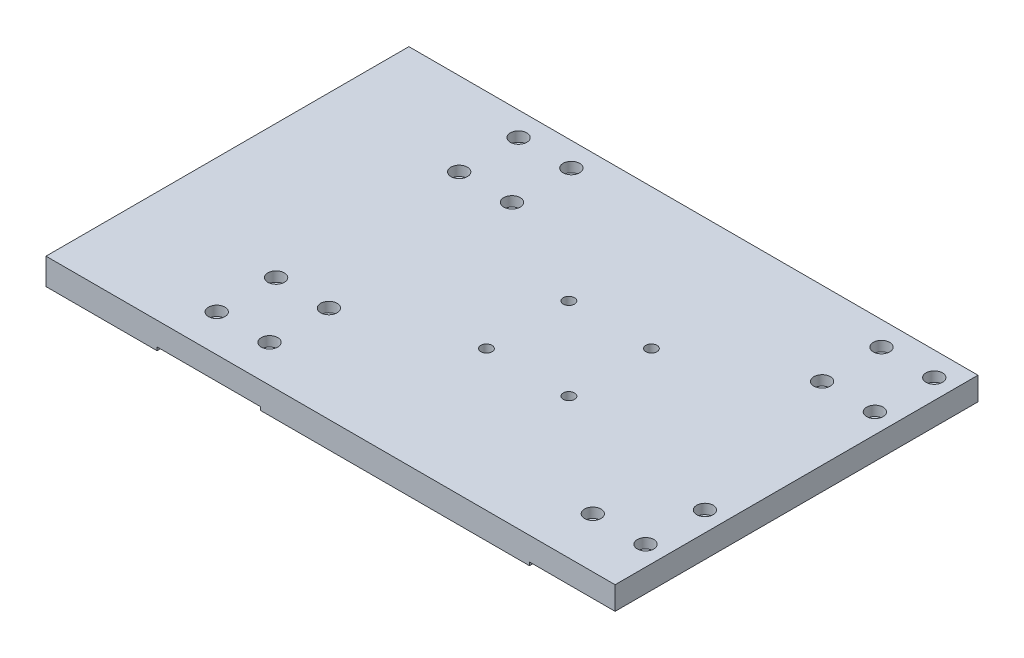
from build123d import *

# Parameters (mm, degrees)
SKETCH1_W                               = 345
SKETCH1_H                               = 220
BOSS_EXTRUDE1_DEPTH                     = 16
CBORE_FOR_M5_HEX_HEAD_BOLT1_D           = 5.5
CBORE_FOR_M5_HEX_HEAD_BOLT1_CBORE_D     = 10
CBORE_FOR_M5_HEX_HEAD_BOLT1_CBORE_DEPTH = 6
SKETCH4_W                               = 62.700686025
SKETCH4_H                               = 220
SKETCH4_W_2                             = 51.921757643
CUT_EXTRUDE1_DEPTH                      = 2
M8_TAPPED_HOLE1_D                       = 6.8


with BuildPart() as part:
    # Sketch1 → Boss-Extrude1 (new body)
    with BuildSketch(Plane(origin=(0, 0, 0), x_dir=(1, 0, 0), z_dir=(0, 1, 0))):
        Rectangle(SKETCH1_W, SKETCH1_H)
    extrude(amount=BOSS_EXTRUDE1_DEPTH)

    # CBORE for M5 Hex Head Bolt1 (through all)
    with Locations(Plane(origin=(0, 16, 0), x_dir=(1, 0, 0), z_dir=(0, 1, 0))):
        with Locations((160.5, 95.483075679), (128.5, 95.483075679), (128.5, 59.483075679), (160.5, 59.483075679), (160.5, -43.516924321), (160.5, -79.516924321), (128.5, -79.516924321), (-91.5, -51.5), (-59.5, -51.5), (-59.5, -87.5), (-91.5, -87.5), (-91.5, 59.483075679), (-59.5, 59.483075679), (-59.5, 95.483075679), (-91.5, 95.483075679)):
            CounterBoreHole(CBORE_FOR_M5_HEX_HEAD_BOLT1_D / 2, CBORE_FOR_M5_HEX_HEAD_BOLT1_CBORE_D / 2, CBORE_FOR_M5_HEX_HEAD_BOLT1_CBORE_DEPTH)

    # Sketch4 → Cut-Extrude1 (cut)
    with BuildSketch(Plane.XZ):
        with Locations((-73.793884323, 0)):
            Rectangle(SKETCH4_W, SKETCH4_H)
        with Locations((146.539121179, 0)):
            Rectangle(SKETCH4_W_2, SKETCH4_H)
    extrude(amount=-CUT_EXTRUDE1_DEPTH, mode=Mode.SUBTRACT)

    # M8 Tapped Hole1 (through all)
    with Locations(Plane(origin=(0, 0, 0), x_dir=(-1, 0, 0), z_dir=(0, -1, 0))):
        with Locations((-59.5, 25), (-9.5, 25), (-9.5, -25), (-59.5, -25)):
            Hole(M8_TAPPED_HOLE1_D / 2)


solid = part.part
